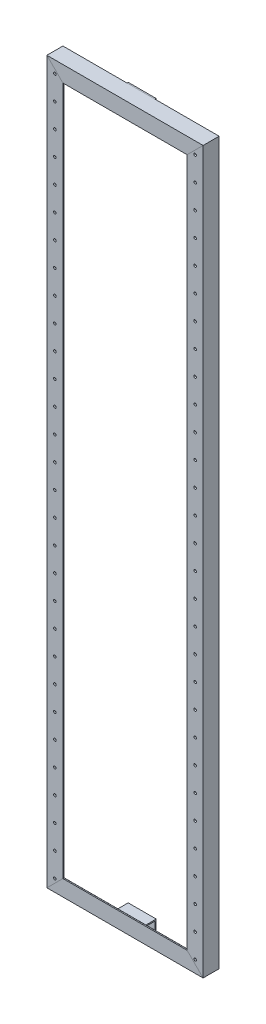
from build123d import *

# Parameters (mm, degrees)
MEMBER_1_DEPTH      = 1857.568542495
MEMBER_1_DEPTH_BACK = 57.568542495
MEMBER_1_2_DEPTH    = 505.13708499
MEMBER_1_3_DEPTH    = 1915.13708499
MEMBER_1_4_DEPTH    = 505.13708499
SKETCH_2_R          = 3.25
CUT_EXTRUDE_1_DEPTH = 4
EXTRUDE_1_DEPTH     = 35
EXTRUDE_1_2_DEPTH   = 35


with BuildPart() as part:
    # Sketch1 → Member 1 (new, two sides: drawn at the far end of the back side and taken through both)
    with BuildSketch(Plane(origin=(195, -900, 0), x_dir=(-1, 0, 0), z_dir=(0, 1, 0)).offset(-MEMBER_1_DEPTH_BACK)):
        with BuildLine():
            Line((40, 0), (0, 0))
            Line((0, 0), (0, -40))
            Line((0, -40), (2.666666667, -40))
            ThreePointArc((2.666666667, -40), (3.609475708, -39.609475708), (4, -38.666666667))
            Line((4, -38.666666667), (4, -9))
            ThreePointArc((4, -9), (5.464466094, -5.464466094), (9, -4))
            Line((9, -4), (38.666666667, -4))
            ThreePointArc((38.666666667, -4), (39.609475708, -3.609475708), (40, -2.666666667))
            Line((40, -2.666666667), (40, 0))
        make_face()
    extrude(amount=MEMBER_1_DEPTH + MEMBER_1_DEPTH_BACK)

    # Member 1 mitre 1
    split(bisect_by=Plane(origin=(195, -900, 0), x_dir=(-0.707106781, 0.707106781, 0), z_dir=(0.707106781, 0.707106781, 0)), keep=Keep.TOP)

    # Member 1 mitre 2
    split(bisect_by=Plane(origin=(195, 900, 0), x_dir=(0.707106781, 0.707106781, 0), z_dir=(0.707106781, -0.707106781, 0)), keep=Keep.TOP)


with BuildPart() as body_2:
    # Sketch1 on segment 2 (carried to segment 2) → Member 1 2 (new body)
    with BuildSketch(Plane(origin=(252.568542495, 900, 0), x_dir=(0, -1, 0), z_dir=(-1, 0, 0))):
        with BuildLine():
            Line((40, 0), (0, 0))
            Line((0, 0), (0, -40))
            Line((0, -40), (2.666666667, -40))
            ThreePointArc((2.666666667, -40), (3.609475708, -39.609475708), (4, -38.666666667))
            Line((4, -38.666666667), (4, -9))
            ThreePointArc((4, -9), (5.464466094, -5.464466094), (9, -4))
            Line((9, -4), (38.666666667, -4))
            ThreePointArc((38.666666667, -4), (39.609475708, -3.609475708), (40, -2.666666667))
            Line((40, -2.666666667), (40, 0))
        make_face()
    extrude(amount=MEMBER_1_2_DEPTH)

    # Member 1 2 mitre 1
    split(bisect_by=Plane(origin=(195, 900, 0), x_dir=(-0.707106781, -0.707106781, 0), z_dir=(-0.707106781, 0.707106781, 0)), keep=Keep.TOP)

    # Member 1 2 mitre 2
    split(bisect_by=Plane(origin=(-195, 900, 0), x_dir=(-0.707106781, 0.707106781, 0), z_dir=(0.707106781, 0.707106781, 0)), keep=Keep.TOP)


with BuildPart() as body_3:
    # Sketch1 on segment 3 (carried to segment 3) → Member 1 3 (new body)
    with BuildSketch(Plane(origin=(-195, 957.568542495, 0), x_dir=(1, 0, 0), z_dir=(0, -1, 0))):
        with BuildLine():
            Line((40, 0), (0, 0))
            Line((0, 0), (0, -40))
            Line((0, -40), (2.666666667, -40))
            ThreePointArc((2.666666667, -40), (3.609475708, -39.609475708), (4, -38.666666667))
            Line((4, -38.666666667), (4, -9))
            ThreePointArc((4, -9), (5.464466094, -5.464466094), (9, -4))
            Line((9, -4), (38.666666667, -4))
            ThreePointArc((38.666666667, -4), (39.609475708, -3.609475708), (40, -2.666666667))
            Line((40, -2.666666667), (40, 0))
        make_face()
    extrude(amount=MEMBER_1_3_DEPTH)

    # Member 1 3 mitre 1
    split(bisect_by=Plane(origin=(-195, -900, 0), x_dir=(-0.707106781, -0.707106781, 0), z_dir=(-0.707106781, 0.707106781, 0)), keep=Keep.TOP)

    # Member 1 3 mitre 2
    split(bisect_by=Plane(origin=(-195, 900, 0), x_dir=(0.707106781, -0.707106781, 0), z_dir=(-0.707106781, -0.707106781, 0)), keep=Keep.TOP)


with BuildPart() as body_4:
    # Sketch1 on segment 4 (carried to segment 4) → Member 1 4 (new body)
    with BuildSketch(Plane(origin=(-252.568542495, -900, 0), x_dir=(0, 1, 0), z_dir=(1, 0, 0))):
        with BuildLine():
            Line((40, 0), (0, 0))
            Line((0, 0), (0, -40))
            Line((0, -40), (2.666666667, -40))
            ThreePointArc((2.666666667, -40), (3.609475708, -39.609475708), (4, -38.666666667))
            Line((4, -38.666666667), (4, -9))
            ThreePointArc((4, -9), (5.464466094, -5.464466094), (9, -4))
            Line((9, -4), (38.666666667, -4))
            ThreePointArc((38.666666667, -4), (39.609475708, -3.609475708), (40, -2.666666667))
            Line((40, -2.666666667), (40, 0))
        make_face()
    extrude(amount=MEMBER_1_4_DEPTH)

    # Member 1 4 mitre 1
    split(bisect_by=Plane(origin=(195, -900, 0), x_dir=(0.707106781, -0.707106781, 0), z_dir=(-0.707106781, -0.707106781, 0)), keep=Keep.TOP)

    # Member 1 4 mitre 2
    split(bisect_by=Plane(origin=(-195, -900, 0), x_dir=(0.707106781, 0.707106781, 0), z_dir=(0.707106781, -0.707106781, 0)), keep=Keep.TOP)


with BuildPart() as cut_extrude_1_tool:
    # 草图2 → 切除-拉伸1 (new body)
    with BuildSketch(Plane.XY):
        with Locations((175, 870)):
            Circle(SKETCH_2_R)
        with Locations(Location((-175, 870, 0), (0, 0, 270))):
            Circle(SKETCH_2_R)
        with Locations(Location((-175, 810, 0), (0, 0, 270))):
            Circle(SKETCH_2_R)
        with Locations((175, 810)):
            Circle(SKETCH_2_R)
        with Locations(Location((-175, 750, 0), (0, 0, 270))):
            Circle(SKETCH_2_R)
        with Locations((175, 750)):
            Circle(SKETCH_2_R)
        with Locations(Location((-175, 690, 0), (0, 0, 270))):
            Circle(SKETCH_2_R)
        with Locations((175, 690)):
            Circle(SKETCH_2_R)
        with Locations(Location((-175, 630, 0), (0, 0, 270))):
            Circle(SKETCH_2_R)
        with Locations((175, 630)):
            Circle(SKETCH_2_R)
        with Locations(Location((-175, 570, 0), (0, 0, 270))):
            Circle(SKETCH_2_R)
        with Locations((175, 570)):
            Circle(SKETCH_2_R)
        with Locations(Location((-175, 510, 0), (0, 0, 270))):
            Circle(SKETCH_2_R)
        with Locations((175, 510)):
            Circle(SKETCH_2_R)
        with Locations(Location((-175, 450, 0), (0, 0, 270))):
            Circle(SKETCH_2_R)
        with Locations((175, 450)):
            Circle(SKETCH_2_R)
        with Locations(Location((-175, 390, 0), (0, 0, 270))):
            Circle(SKETCH_2_R)
        with Locations((175, 390)):
            Circle(SKETCH_2_R)
        with Locations(Location((-175, 330, 0), (0, 0, 270))):
            Circle(SKETCH_2_R)
        with Locations((175, 330)):
            Circle(SKETCH_2_R)
        with Locations(Location((-175, 270, 0), (0, 0, 270))):
            Circle(SKETCH_2_R)
        with Locations((175, 270)):
            Circle(SKETCH_2_R)
        with Locations(Location((-175, 210, 0), (0, 0, 270))):
            Circle(SKETCH_2_R)
        with Locations((175, 210)):
            Circle(SKETCH_2_R)
        with Locations(Location((-175, 150, 0), (0, 0, 270))):
            Circle(SKETCH_2_R)
        with Locations((175, 150)):
            Circle(SKETCH_2_R)
        with Locations(Location((-175, 90, 0), (0, 0, 270))):
            Circle(SKETCH_2_R)
        with Locations((175, 90)):
            Circle(SKETCH_2_R)
        with Locations(Location((-175, 30, 0), (0, 0, 270))):
            Circle(SKETCH_2_R)
        with Locations((175, 30)):
            Circle(SKETCH_2_R)
        with Locations(Location((-175, -30, 0), (0, 0, 270))):
            Circle(SKETCH_2_R)
        with Locations((175, -30)):
            Circle(SKETCH_2_R)
        with Locations(Location((-175, -90, 0), (0, 0, 270))):
            Circle(SKETCH_2_R)
        with Locations((175, -90)):
            Circle(SKETCH_2_R)
        with Locations(Location((-175, -150, 0), (0, 0, 270))):
            Circle(SKETCH_2_R)
        with Locations((175, -150)):
            Circle(SKETCH_2_R)
        with Locations(Location((-175, -210, 0), (0, 0, 270))):
            Circle(SKETCH_2_R)
        with Locations((175, -210)):
            Circle(SKETCH_2_R)
        with Locations(Location((-175, -270, 0), (0, 0, 270))):
            Circle(SKETCH_2_R)
        with Locations((175, -270)):
            Circle(SKETCH_2_R)
        with Locations(Location((-175, -330, 0), (0, 0, 270))):
            Circle(SKETCH_2_R)
        with Locations((175, -330)):
            Circle(SKETCH_2_R)
        with Locations(Location((-175, -390, 0), (0, 0, 270))):
            Circle(SKETCH_2_R)
        with Locations((175, -390)):
            Circle(SKETCH_2_R)
        with Locations(Location((-175, -450, 0), (0, 0, 270))):
            Circle(SKETCH_2_R)
        with Locations((175, -450)):
            Circle(SKETCH_2_R)
        with Locations(Location((-175, -510, 0), (0, 0, 270))):
            Circle(SKETCH_2_R)
        with Locations((175, -510)):
            Circle(SKETCH_2_R)
        with Locations(Location((-175, -570, 0), (0, 0, 270))):
            Circle(SKETCH_2_R)
        with Locations((175, -570)):
            Circle(SKETCH_2_R)
        with Locations(Location((-175, -630, 0), (0, 0, 270))):
            Circle(SKETCH_2_R)
        with Locations((175, -630)):
            Circle(SKETCH_2_R)
        with Locations(Location((-175, -690, 0), (0, 0, 270))):
            Circle(SKETCH_2_R)
        with Locations((175, -690)):
            Circle(SKETCH_2_R)
        with Locations(Location((-175, -750, 0), (0, 0, 270))):
            Circle(SKETCH_2_R)
        with Locations((175, -750)):
            Circle(SKETCH_2_R)
        with Locations(Location((-175, -810, 0), (0, 0, 270))):
            Circle(SKETCH_2_R)
        with Locations((175, -810)):
            Circle(SKETCH_2_R)
        with Locations(Location((-175, -870, 0), (0, 0, 270))):
            Circle(SKETCH_2_R)
        with Locations((175, -870)):
            Circle(SKETCH_2_R)
    extrude(amount=-CUT_EXTRUDE_1_DEPTH)


with BuildPart() as part_1:
    add(part.part)

    # 切除-拉伸1: cut by cut_extrude_1_tool
    add(cut_extrude_1_tool.part, mode=Mode.SUBTRACT)


with BuildPart() as body_3_1:
    add(body_3.part)

    # 切除-拉伸1: cut by cut_extrude_1_tool
    add(cut_extrude_1_tool.part, mode=Mode.SUBTRACT)


with BuildPart() as body_5:
    # 草图3 → 凸台-拉伸1 (new, symmetric)
    with BuildSketch(Plane(origin=(0, 0, 0), x_dir=(0, 0, -1), z_dir=(1, 0, 0))):
        Polygon((3, -874), (3, -877), (40, -877), (40, -900), (43, -900), (43, -874), align=None)
    extrude(amount=EXTRUDE_1_DEPTH, both=True)


with BuildPart() as body_6:
    # 草图3 → Extrude 1 2 (new, symmetric)
    with BuildSketch(Plane(origin=(0, 0, 0), x_dir=(0, 0, -1), z_dir=(1, 0, 0))):
        Polygon((3, 874), (43, 874), (43, 900), (40, 900), (40, 877), (3, 877), align=None)
    extrude(amount=EXTRUDE_1_2_DEPTH, both=True)


solid = Compound([body_2.part, body_4.part, part_1.part, body_3_1.part, body_5.part, body_6.part])
